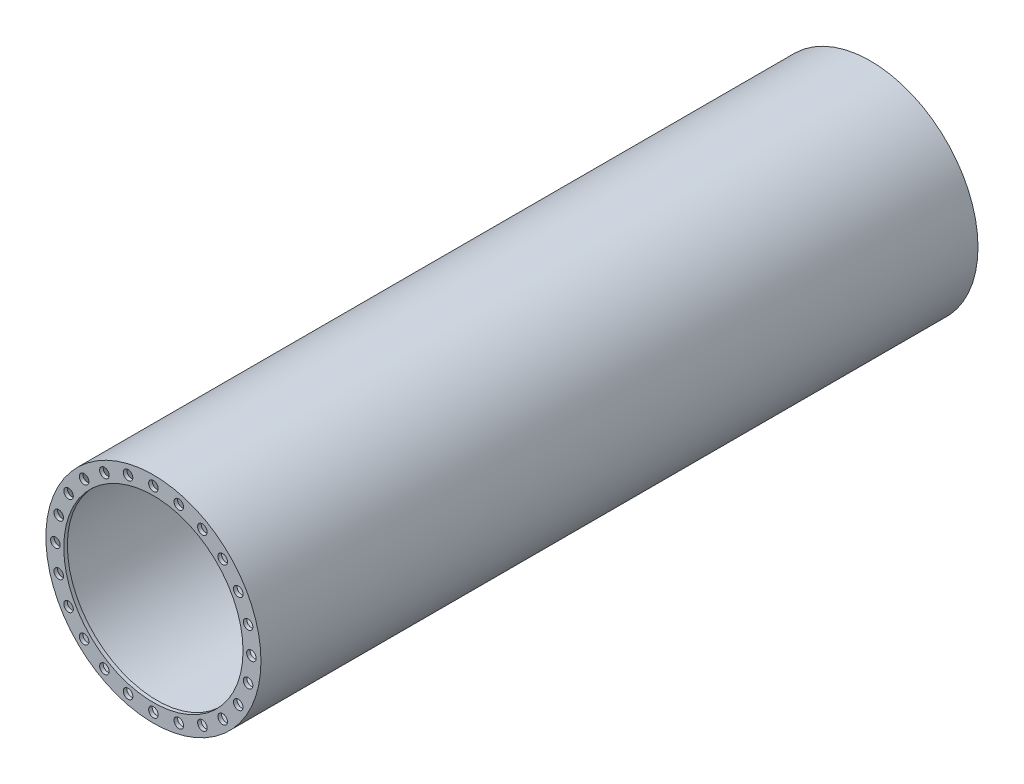
SolidWorks part; units mm, degrees
ref_plane "前视基准面" through (0, 0, 0) normal (0, 0, 1) x (1, 0, 0)
ref_plane "上视基准面" through (0, 0, 0) normal (0, 1, 0) x (1, 0, 0)
ref_plane "右视基准面" through (0, 0, 0) normal (1, 0, 0) x (0, 0, -1)
other "Configuration Table"
sketch "草图1" plane through (0, 0, 0) normal (0, 0, 1) x (1, 0, 0)
  circle A0 centre (0, 0) radius 450
  circle A1 centre (0, 0) radius 442
  dimension "D1" = 884
  dimension "D2" = 900
extrude "凸台-拉伸1" add sketch "草图1" along normal mid plane 3000
sketch "草图2" plane through (0, 0, 1500) normal (0, 0, 1) x (1, 0, 0)
  circle A0 centre (0, 0) radius 450 construction
  circle A1 centre (0, 0) radius 450
  circle A2 centre (0, 0) radius 375
  dimension "D1" = 750
extrude "凸台-拉伸3" add sketch "草图2" against normal blind 15
mirror "镜向1" about plane through (0, 0, 0) normal (0, 0, 1) of "凸台-拉伸3"
sketch "草图3" plane through (0, 0, 1500) normal (0, 0, 1) x (1, 0, 0)
  circle A0 centre (0, 0) radius 410 construction
  circle A1 centre (0, 410) radius 20
  circle A2 centre (106.1158, 396.0296) radius 20
  circle A3 centre (205, 355.0704) radius 20
  circle A4 centre (289.9138, 289.9138) radius 20
  circle A5 centre (355.0704, 205) radius 20
  circle A6 centre (396.0296, 106.1158) radius 20
  circle A7 centre (410, 0) radius 20
  circle A8 centre (396.0296, -106.1158) radius 20
  circle A9 centre (355.0704, -205) radius 20
  circle A10 centre (289.9138, -289.9138) radius 20
  circle A11 centre (205, -355.0704) radius 20
  circle A12 centre (106.1158, -396.0296) radius 20
  circle A13 centre (0, -410) radius 20
  circle A14 centre (-106.1158, -396.0296) radius 20
  circle A15 centre (-205, -355.0704) radius 20
  circle A16 centre (-289.9138, -289.9138) radius 20
  circle A17 centre (-355.0704, -205) radius 20
  circle A18 centre (-396.0296, -106.1158) radius 20
  circle A19 centre (-410, 0) radius 20
  circle A20 centre (-396.0296, 106.1158) radius 20
  circle A21 centre (-355.0704, 205) radius 20
  circle A22 centre (-289.9138, 289.9138) radius 20
  circle A23 centre (-205, 355.0704) radius 20
  circle A24 centre (-106.1158, 396.0296) radius 20
  dimension "D1" = 820
  dimension "D2" = 40
  dimension "D3" = 24
extrude "切除-拉伸1" cut sketch "草图3" against normal through all
